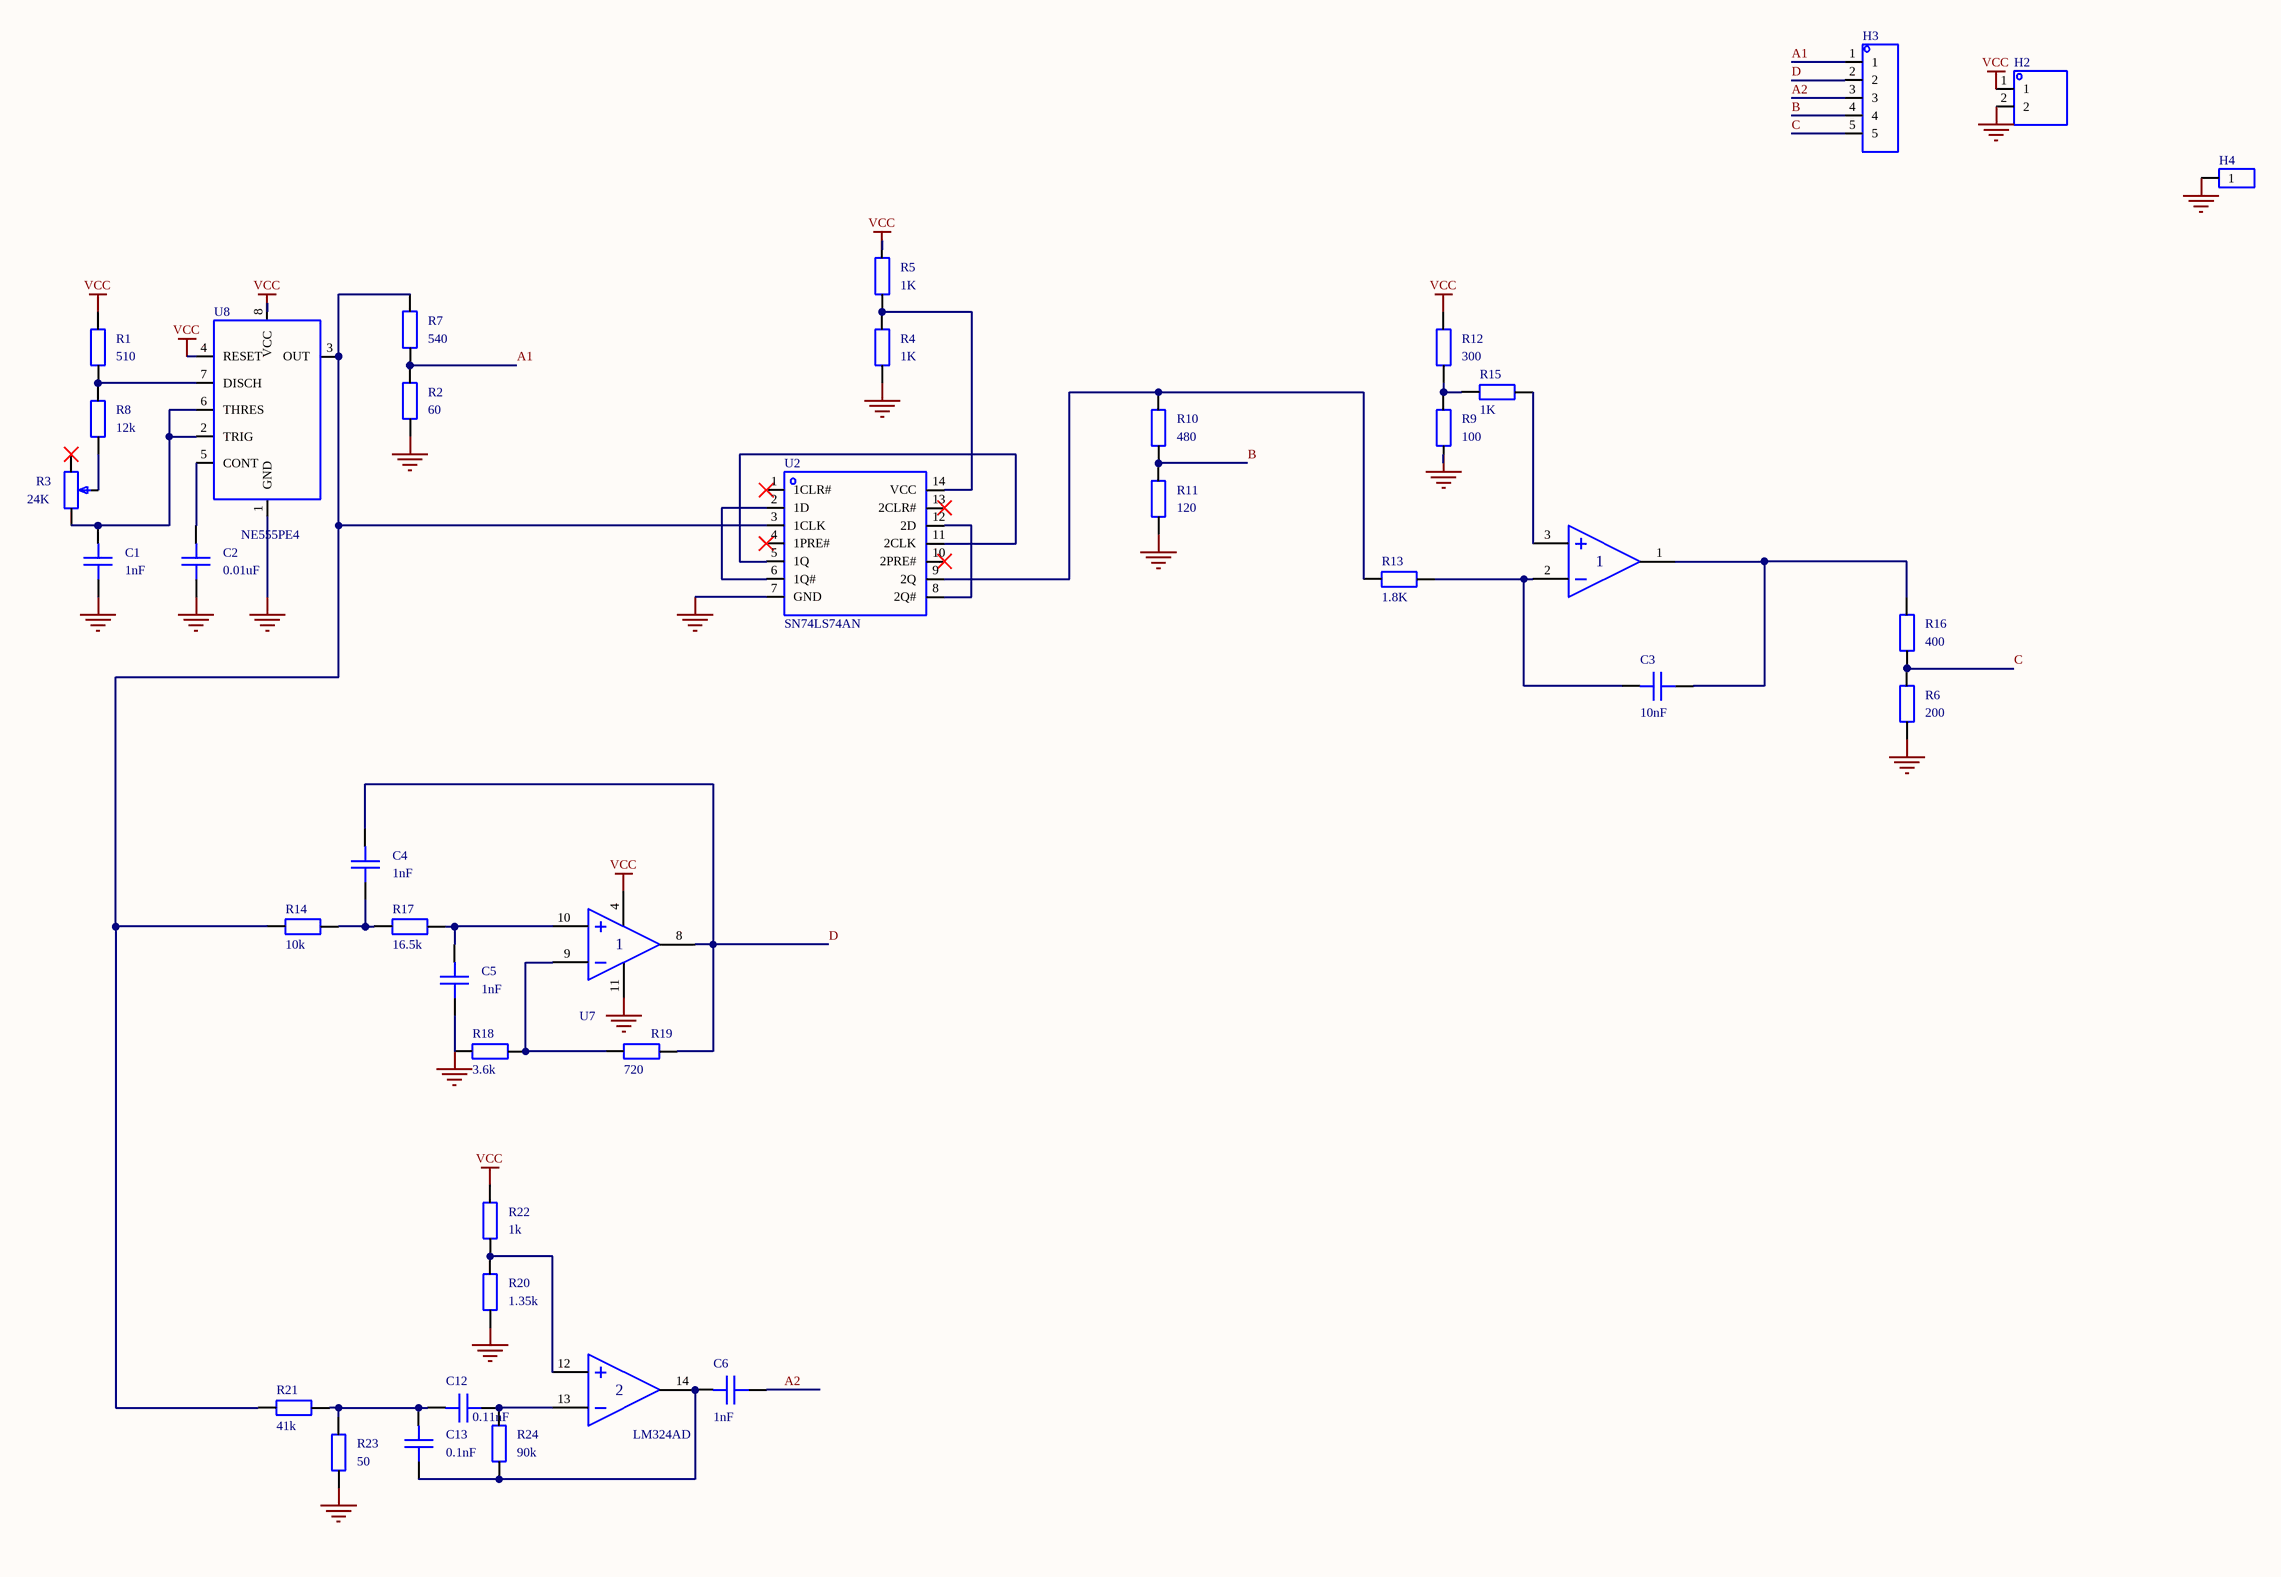
[diagram p0: MISC49933-3.schdoc]
# Altium project MISC49933-2.PrjPcb
1 sheet, 38 parts. Net scope: global (net labels, ports and power ports of the same name join across sheets).
Board file: MISC49933.pcbdoc

## Sheet MISC49933-3.schdoc
size 178 x 98 mm; Version: V1.0; @Project Name: MISC49933; @Page Count: 1; @Update Date: 2024-12-09; @Create Date: 2024-12-09; @Schematic Name: MISC49933; @Page No: 1; @Board Name: MISC49933; @Create Time: 12:10:11; @Update Time: 21:07:45

### Parts
C1  1nF  [C0805]
C2  0.01uF  [C0805]
C3  10nF  [C0805]
C4  1nF  [C0805]
C5  1nF  [C0805]
C6  1nF  [C0805]
C12  0.11nF  [C0805]
C13  0.1nF  [C0805]
H2  (no value)  [HDR-TH_2P-P2.54-V-M-1]
H3  (no value)  [HDR-TH_5P-P2.54-V-M]
H4  (no value)  [HDR-TH_1P-V-M_XKB_X4611WV-01I-C28D40]
R1  510  [R0603]
R2  60  [R0603]
R3  24K  [R_3296]
R4  1K  [R0603]
R5  1K  [R0603]
R6  200  [R0603]
R7  540  [R0603]
R8  12k  [R0603]
R9  100  [R0603]
R10  480  [R0603]
R11  120  [R0603]
R12  300  [R0603]
R13  1.8K  [R0603]
R14  10k  [R0603]
R15  1K  [R0603]
R16  400  [R0603]
R17  16.5k  [R0603]
R18  3.6k  [R0603]
R19  720  [R0603]
R20  1.35k  [R0603]
R21  41k  [R0603]
R22  1k  [R0603]
R23  50  [R0603]
R24  90k  [R0603]
U2  SN74LS74AN  [PDIP-14_L19.5-W6.7-P2.54-LS7.9-BL]
U7  LM324AD  [SOIC-14_L8.7-W3.9-P1.27-LS6.0-BL]
U8  NE555PE4  [PDIP-8_L9.6-W6.4-P2.54-LS7.9-BL-1]

### Nets
GND: C1.1 C2.1 C5.1 H2.2 H4.1 R2.1 R4.1 R6.1 R9.2 R11.1 R18.2 R20.2 R23.2 U2.7(GND) U7.11(GND) U8.1(GND)
VCC: H2.1 R1.2 R5.2 R12.1 R22.1 U7.4(VCC) U8.4(RESET) U8.8(VCC)
A1: H3.1 R2.2 R7.1
A2: C6.1 H3.3
B: H3.4 R10.1 R11.2
C: H3.5 R6.2 R16.1
D: C4.2 H3.2 R19.1 U7.8(1OUT)
NetC1_2: C1.2 R3.1 U8.2(TRIG) U8.6(THRES)
NetC2_2: C2.2 U8.5(CONT)
NetC3_1: C3.1 R16.2 U7.1(1OUT)
NetC3_2: C3.2 R13.1 U7.2(1IN+)
NetC4_1: C4.1 R14.1 R17.2
NetC5_2: C5.2 R17.1 U7.10(1IN-)
NetC6_2: C6.2 C13.1 R24.2 U7.14(1OUT)
NetC12_1: C12.1 R24.1 U7.13(1IN+)
NetC12_2: C12.2 C13.2 R21.1 R23.1
NetR1_1: R1.1 R8.2 U8.7(DISCH)
NetR3_2: R3.2 R8.1
NetR4_2: R4.2 R5.1 U2.14(VCC)
NetR7_2: R7.2 R14.2 R21.2 U2.3(1CLK) U8.3(OUT)
NetR9_1: R9.1 R12.2 R15.2
NetR10_2: R10.2 R13.2 U2.9(2Q)
NetR15_1: R15.1 U7.3(1IN-)
NetR18_1: R18.1 R19.2 U7.9(1IN+)
NetR20_1: R20.1 R22.2 U7.12(1IN-)
NetU2_2: U2.2(1D) U2.6(1Q#)
NetU2_5: U2.5(1Q) U2.11(2CLK)
NetU2_8: U2.8(2Q#) U2.12(2D)

Not connected (* = marked no-connect by the designer): R3 3*; U2 1(1CLR#)* 4(1PRE#)* 10(2PRE#)* 13(2CLR#)*

### Notes on the sheet
- 2024-12-09
- Schematic
- Sheet
- Item code
- P1
- Reviewed
- Drawn
- Revision
- Size
- page
- Total
- A4
- 1

### Library data of the parts
C1-C6 C12 C13 = CAP_0805: ConvertToPcb: yes; SymbolName: CapAcitance; ModelId: 1ba041120af144c991958decab20d241; ModelName: C0805_L2.0-W1.3-H1.3; ModelTransform: 78.74,51.181,0,0,0,0,0,0.0005,0; Device: CAP_0805; AddInBom: yes; Supplier Footprint: 0805; FootprintName: C0805
  C1 C4-C6: Value: 1nF
  C2: Value: 0.01uF
  C3: Value: 10nF
  C12: Value: 0.11nF
  C13: Value: 0.1nF
H2 = HDR-M_2.54_1x2P: Symbol: 210S-1*2P L=11.6MMGold-plated black; ConvertToPcb: yes; ModelId: 79b2e9f2d70a4d68a1b7098f27c6d4c5; ModelName: HDR-M-2.54_1x2; ModelTransform: 200,100,0,0,0,0,0,0,-118.11; Device: HDR-M_2.54_1x2P; AddInBom: yes; SupplierPart: C124375; Supplier Footprint: 插件; FootprintName: HDR-TH_2P-P2.54-V-M-1
H3 = HDR-M_2.54_1x5P: Symbol: MTP125-1105S1; ConvertToPcb: yes; ModelId: 47d466e4a34f4fc5bc626cf773a24dd5; ModelName: HDR-TH_5P-P2.54-M-LI-1X5P; ModelTransform: 499.999,100,0,0,0,0,0,0,-118.11; Device: HDR-M_2.54_1x5P; AddInBom: yes; SupplierPart: C358687; Supplier Footprint: 插件; FootprintName: HDR-TH_5P-P2.54-V-M
H4 = HDR-M_2.54_1x1P: Symbol: HDR_1x1; ConvertToPcb: yes; ModelId: 95857080d3cc4057a19a22ccce05e171; ModelTransform: 78.74,79.1337,0,0,0,0,0,0,-110.236; Device: HDR-M_2.54_1x1P; AddInBom: yes; SupplierPart: C81276; Supplier Footprint: 插件; FootprintName: HDR-TH_1P-V-M_XKB_X4611WV-01I-C28D40; JLCPCB Part Class: Extended Part; ModelName: HDR-TH_1P-V-M_XKB_X4611WV-01I-C28D40
R1 R2 R4-R24 = Res_0603: Symbol: Resistor; ConvertToPcb: yes; ModelId: fc143cca1e79419f9cd78b61e9279f08; ModelTransform: 31.8897,63.7794,0,90,0,0,0,0,0; Device: Res_0603; AddInBom: yes; Supplier Footprint: 0603; FootprintName: R0603; ModelName: R0603
  R1: Value: 510
  R2: Value: 60
  R4 R5 R15: Value: 1K
  R6: Value: 200
  R7: Value: 540
  R8: Value: 12k
  R9: Value: 100
  R10: Value: 480
  R11: Value: 120
  R12: Value: 300
  R13: Value: 1.8K
  R14: Value: 10k
  R16: Value: 400
  R17: Value: 16.5k
  R18: Value: 3.6k
  R19: Value: 720
  R20: Value: 1.35k
  R21: Value: 41k
  R22: Value: 1k
  R23: Value: 50
  R24: Value: 90k
R3 = R_3296: ConvertToPcb: yes; ModelId: b182808559bb43bda9e7de64b64134cb; ModelName: 3296W; ModelTransform: 373.98,188.96,590.49,180,0,0,0,0,-140; Value: 24K; Device: R_3296; AddInBom: yes; Supplier Footprint: 直插; SymbolName: R_3296; FootprintName: R_3296
U2 = SN74LS74AN: Type: D-type; supply voltage: 4.75V~5.25V; clock frequency: 33MHz; number of elements: 2; bits per element: 1; max propagation delay: 25ns@2.5V,15pF; quiescent current (Iq): 8mA;; Manufacturer: TI(德州仪器); AddInBom: yes; ModelId: 54e4a14e1c964e4d8957b52ed5aa85d9; ModelTransform: 767.715,311.023,0,0,0,0,0,0,-129.921; Trigger Type: Rising edge; Function: Set and reset; Number of Elements: 2; Number of Bits per Element: 1; Output Type: Complementary; Source Current: 400uA; Symbol: SN74LS74AN; Device: SN74LS74AN; LCSC Part Name: SN74LS74AN; SupplierPart: C1523173; ManufacturerPart: SN74LS74AN; Supplier Footprint: PDIP-14; Supplier: LCSC; ConvertToPcb: yes; FootprintName: PDIP-14_L19.5-W6.7-P2.54-LS7.9-BL; ModelName: PDIP-14_L19.5-W6.7-P2.54-LS7.9-BL; Supply Voltage: 4.75V~5.25V; Clock Frequency: 33MHz; Maximum Propagation Delay: 25ns@2.5V,15pF; Series: 74LS series; Sink Current: 8mA; Quiescent Current (Iq): 8mA; Input Capacitance: -; Operating Temperature: 0℃~+70℃
U7 = LM324AD: Amplifier count: quad; gain-bandwidth product (GBP): 1.3MHz; input bias current (Ib): 15nA; slew rate (SR): 0.5V/us; bandwidth (-3db): -;; Manufacturer: TI(德州仪器); AddInBom: yes; Output Current: 30mA; ModelId: 8dbf5b715d42428c85558507ae5a252b; ModelName: SOIC-14_L8.6-W3.9-H1.8-LS6.0-P1.27; ModelTransform: 338.583,236.22,0,0,0,0,0,-0.001,0; Symbol: LM324AD; Device: LM324AD; LCSC Part Name: LM324AD; SupplierPart: C1346258; ManufacturerPart: LM324AD; Supplier Footprint: SOIC-14; JLCPCB Part Class: Extended library; Supplier: LCSC; ConvertToPcb: yes; Number of Circuits: Quad; Gain Bandwidth Product(GBP): 1.3MHz; Current - Input Bias(Ib): 15nA; Slew Rate(SR): 0.5V/us; -3db Bandwidth: -; Operating Temperature: 0℃~+70℃; FootprintName: SOIC-14_L8.7-W3.9-P1.27-LS6.0-BL
U8 = NE555PE4: Single-precision timer 8-PDIP 0 to 70; Manufacturer: TI(德州仪器); AddInBom: yes; ModelId: 1b8eaf096e7944deafe216467068c10e; ModelTransform: 377.952,318.897,0,0,0,0,0,0,-118.11; Symbol: NE555PE4; Device: NE555PE4; LCSC Part Name: NE555PE4; SupplierPart: C2859604; ManufacturerPart: NE555PE4; Supplier Footprint: PDIP-8; Supplier: LCSC; ConvertToPcb: yes; FootprintName: PDIP-8_L9.6-W6.4-P2.54-LS7.9-BL-1; ModelName: PDIP-8_L9.6-W6.4-P2.54-LS7.9-BL-1